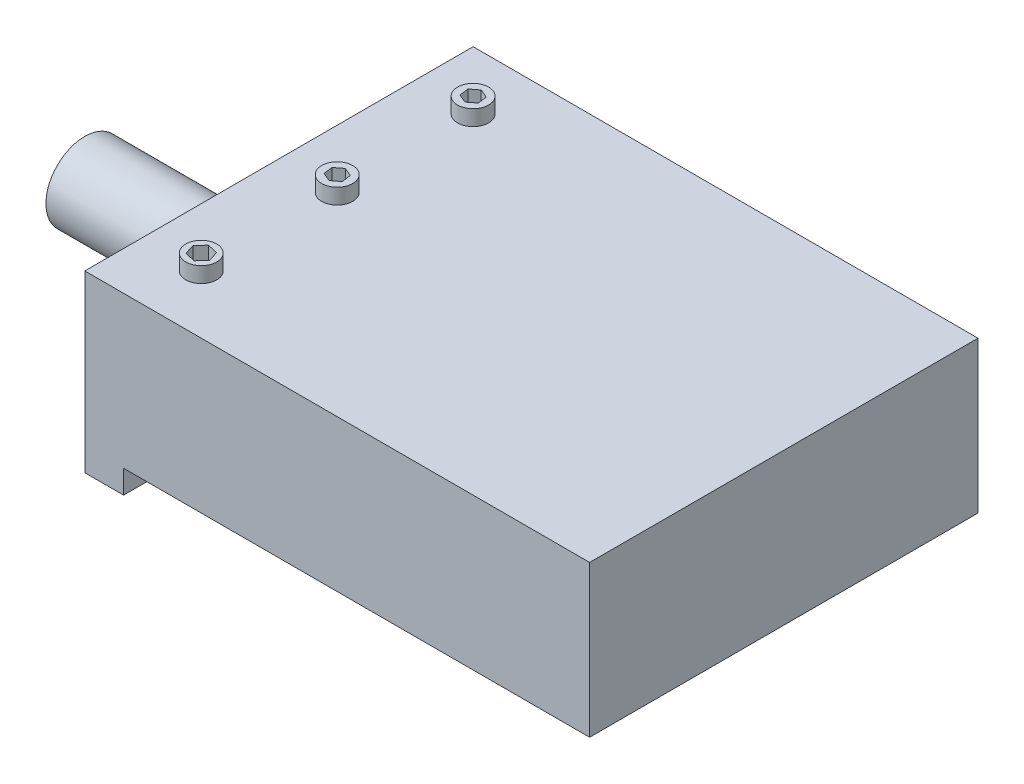
SolidWorks part; units mm, degrees
ref_plane "Front Plane" through (0, 0, 0) normal (0, 0, 1) x (1, 0, 0)
ref_plane "Top Plane" through (0, 0, 0) normal (0, 1, 0) x (1, 0, 0)
ref_plane "Right Plane" through (0, 0, 0) normal (1, 0, 0) x (0, 0, -1)
other "Configuration Table"
sketch "Sketch1" plane through (0, 0, 0) normal (0, 1, 0) x (1, 0, 0)
  line L1 (-35, 50) -> (35, 50)
  line L2 (-35, 50) -> (-35, -50)
  line L3 (-35, -50) -> (35, -50)
  line L4 (35, 50) -> (35, -50)
  line L5 (-35, 50) -> (35, -50) construction
  line L6 (-35, -50) -> (35, 50) construction
  point P0 (0, 0)
  dimension "D1" = 70
  dimension "D2" = 100
extrude "Boss-Extrude1" add sketch "Sketch1" along normal blind 30
sketch "Sketch2" plane through (0, 30, 0) normal (0, 1, 0) x (1, 0, 0)
  line L0 (20, 50) -> (20, -35) construction
  line L1 (35, 50) -> (-35, 50) construction
  line L2 (20, -35) -> (-35, -35) construction
  line L3 (-35, 50) -> (-35, -50) construction
  line L4 (35, -50) -> (35, 50) construction
  line L5 (-35, -50) -> (35, -50) construction
  line L7 (21.9131, 33.5347) -> (22.2255, 35.9241)
  line L8 (22.2255, 35.9241) -> (20.3125, 37.3894)
  line L9 (20.3125, 37.3894) -> (18.0869, 36.4653)
  line L10 (18.0869, 36.4653) -> (17.7745, 34.0759)
  line L11 (17.7745, 34.0759) -> (19.6875, 32.6106)
  line L12 (19.6875, 32.6106) -> (21.9131, 33.5347)
  line L13 (21.9131, -1.4702) -> (22.2298, 0.9217)
  line L14 (22.2298, 0.9217) -> (20.3167, 2.3919)
  line L15 (20.3167, 2.3919) -> (18.0869, 1.4702)
  line L16 (18.0869, 1.4702) -> (17.7702, -0.9217)
  line L17 (17.7702, -0.9217) -> (19.6833, -2.3919)
  line L18 (19.6833, -2.3919) -> (21.9131, -1.4702)
  line L19 (21.9131, -37.0352) -> (22.719, -34.3608)
  line L20 (22.719, -34.3608) -> (20.806, -32.3257)
  line L21 (20.806, -32.3257) -> (18.0869, -32.9648)
  line L22 (18.0869, -32.9648) -> (17.281, -35.6392)
  line L23 (17.281, -35.6392) -> (19.194, -37.6743)
  line L24 (19.194, -37.6743) -> (21.9131, -37.0352)
  circle A1 centre (20, -35) radius 4
  circle A2 centre (20, 0) radius 4
  circle A3 centre (20, 35) radius 4
  circle A4 centre (20, 35) radius 2.0869 construction
  circle A5 centre (20, 0) radius 2.0895 construction
  circle A6 centre (20, -35) radius 2.4189 construction
  dimension "D4" = 8
  dimension "D5" = 8
  dimension "D6" = 8
  dimension "D1" = 15
  dimension "D2" = 15
  dimension "D8" = 35
  dimension "D9" = 35
extrude "Boss-Extrude2" add sketch "Sketch2" along normal blind 4
sketch "Sketch3" plane through (35, 0, 0) normal (1, 0, 0) x (0, 0, -1)
  line L0 (-50, 30) -> (50, 30) construction
  circle A0 centre (0, 0) radius 10
  dimension "D1" = 20
  dimension "D2" = 30
extrude "Boss-Extrude3" add sketch "Sketch3" along normal blind 50
sketch "Sketch4" plane through (0, 0, 0) normal (0, -1, 0) x (1, 0, 0)
  line L1 (-35, 50) -> (35, 50)
  line L2 (-35, 50) -> (-35, -50)
  line L3 (-35, -50) -> (35, -50)
  line L4 (35, 50) -> (35, -50)
extrude "Boss-Extrude4" add sketch "Sketch4" along normal blind 15
mirror "Mirror1" about plane through (-35, 30, -50) normal (1, 0, 0) of bodies 114
ref_plane "Plane1" through (-35, 0, 0) normal (-1, 0, 0) x (0, 0, 1)
sketch "Sketch5" plane through (-35, 0, 0) normal (-1, 0, 0) x (0, 0, 1)
  line L1 (-66.3518, 43.0683) -> (67.899, 43.0683)
  line L2 (-66.3518, 43.0683) -> (-66.3518, -21.7957)
  line L3 (-66.3518, -21.7957) -> (67.899, -21.7957)
  line L4 (67.899, 43.0683) -> (67.899, -21.7957)
extrude "Cut-Extrude1" cut sketch "Sketch5" against normal blind 130
sketch "Sketch6" plane through (0, 0, 50) normal (0, 0, 1) x (1, 0, 0)
  line L0 (-35, 24.75) -> (-35, -24.75) construction
  line L1 (-35, -15) -> (-95, -15)
  line L2 (-35, -15) -> (-35, -9)
  line L3 (-35, -9) -> (-95, -9)
  line L4 (-95, -15) -> (-95, -9)
  line L5 (-35, -15) -> (-105, -15) construction
  dimension "D1" = 60
  dimension "D2" = 6
extrude "Cut-Extrude2" cut sketch "Sketch6" against normal up to next
sketch "Sketch7" plane through (-35, 0, 0) normal (1, 0, 0) x (0, 0, -1)
  line L1 (-50, 30) -> (50, 30)
  line L2 (-50, 30) -> (-50, -9)
  line L3 (-50, -9) -> (50, -9)
  line L4 (50, 30) -> (50, -9)
extrude "Boss-Extrude5" add sketch "Sketch7" along normal blind 60
